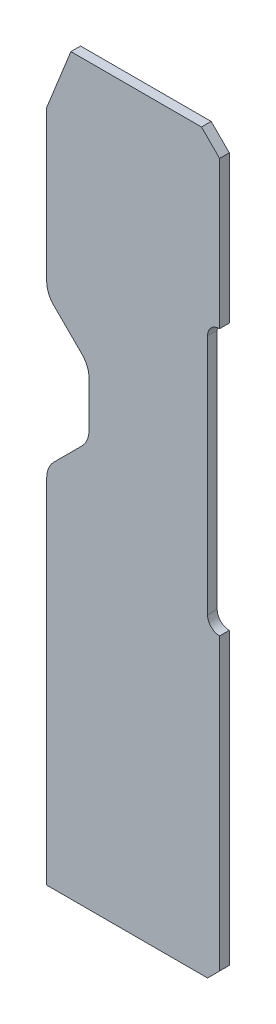
from build123d import *

# Parameters (mm, degrees)
BOSS_EXTRUDE1_DEPTH = 8


with BuildPart() as part:
    # Sketch1 → Boss-Extrude1 (new body)
    with BuildSketch(Plane.XY):
        with BuildLine():
            Line((0, 0), (0, 291.715728753))
            ThreePointArc((0, 291.715728753), (1.52240935, 299.3693974), (5.857864376, 305.857864376))
            Line((5.857864376, 305.857864376), (29.142135624, 329.142135624))
            ThreePointArc((29.142135624, 329.142135624), (33.47759065, 335.6306026), (35, 343.284271247))
            Line((35, 343.284271247), (35, 380.715728753))
            ThreePointArc((35, 380.715728753), (33.47759065, 388.3693974), (29.142135624, 394.857864376))
            Line((29.142135624, 394.857864376), (5.857864376, 418.142135624))
            ThreePointArc((5.857864376, 418.142135624), (1.52240935, 424.6306026), (0, 432.284271247))
            Line((0, 432.284271247), (0, 557))
            Line((0, 557), (20, 607))
            Line((20, 607), (128, 607))
            Line((128, 607), (143, 592))
            Line((143, 592), (143, 470))
            ThreePointArc((143, 470), (135.928932188, 467.071067812), (133, 460))
            Line((133, 460), (133, 260))
            ThreePointArc((133, 260), (135.928932188, 252.928932188), (143, 250))
            Line((143, 250), (143, 10))
            Line((143, 10), (133, 0))
            Line((133, 0), (0, 0))
        make_face()
    extrude(amount=BOSS_EXTRUDE1_DEPTH)


solid = part.part
